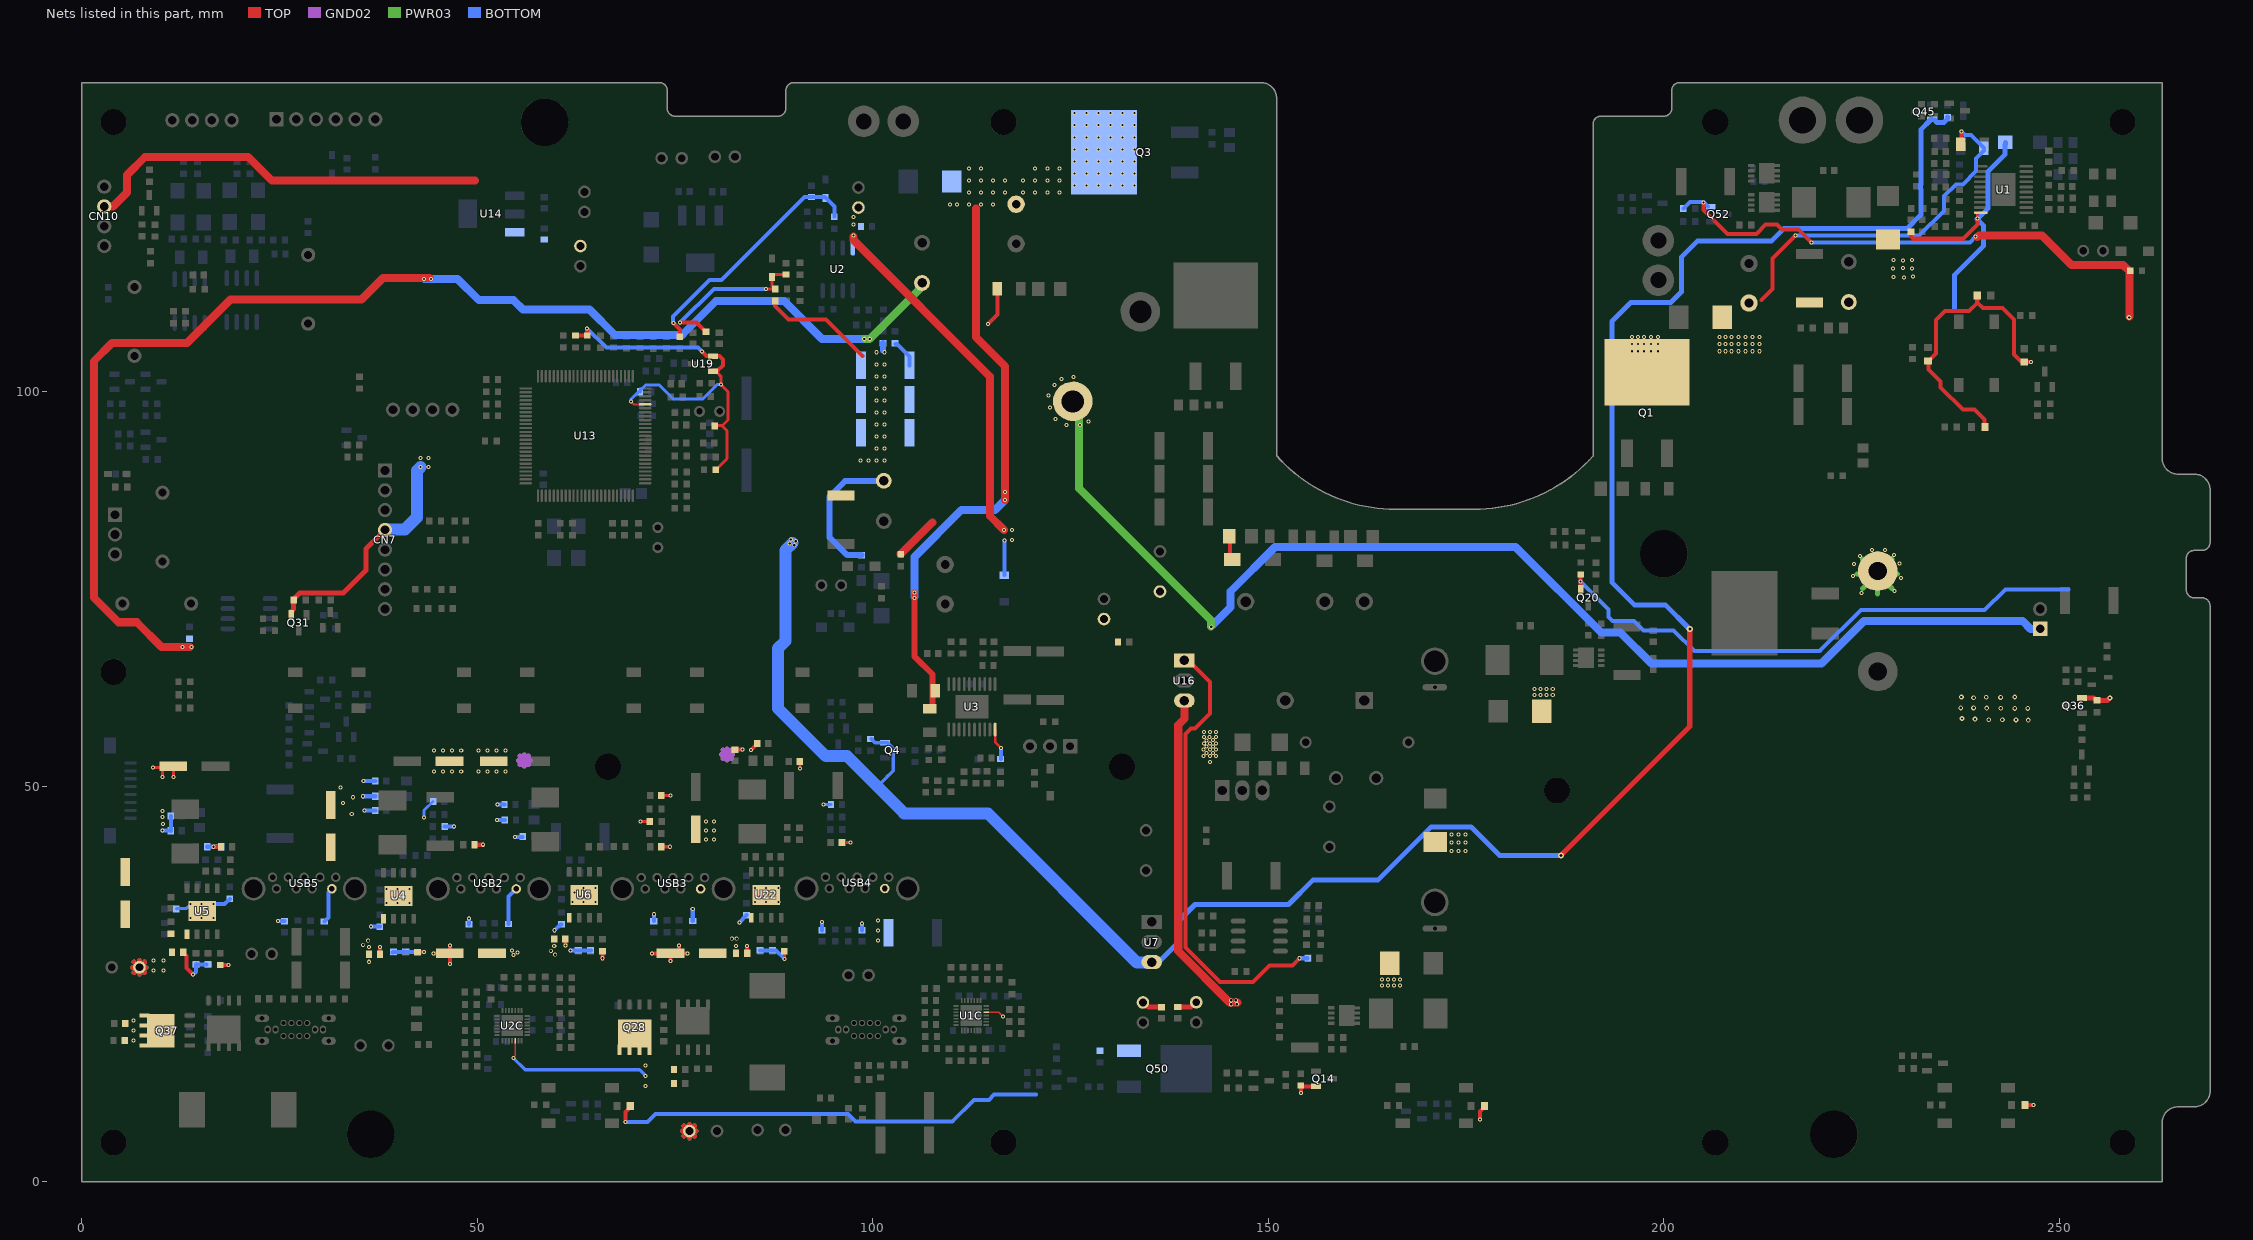
[diagram p0: the nets of this part, all layers, seen from the top]
# Altium PCB MISC84402.PcbDoc (part 3 of 12)
Units mm, origin at the board's own origin, x right, y up, seen from the top; angles counter-clockwise.
Board outline 269.06 x 139 mm, 4 copper layers (TOP, GND02, PWR03, BOTTOM), stack 0.732 mm thick; 694 components, 428 nets, 1859 pads, 1384 vias.

## Footprints (in the part's own frame and the unit in brackets; to place one, negate y for a bottom-side part, rotate by r counter-clockwise, add the part's x,y. Pads: shape width x height; smd on the part's side, far side on the other; paste and mask are expansions set on the pad) (continued)
SOD-123FL_L2.7-W1.8-LS3.8-RD [mm]
  rect 1.4x1.2 smd: 1(-1.735,0) 2(1.735,0)
  silkscreen extent -1.6,-1 1.38,1
SOD-323_L1.8-W1.3-LS2.5-RD [mm]
  rect 1x0.75 smd: 1(-1.173,0) 2(1.173,0)
  silkscreen extent -1.08,-0.8 0.9,0.8
SOIC-8_L5.0-W4.0-P1.27-LS6.0-BL [mm]
  oval 0.568x1.95 smd: 1(-2.59,-1.623) 2(-1.32,-1.623) 3(-0.05,-1.623) 4(1.22,-1.623) 5(1.22,3.787) 6(-0.05,3.787) 7(-1.32,3.787) 8(-2.59,3.787)
  silkscreen extent -3.38,-1.73 1.81,2.99
SOP-8_L4.9-W3.9-P1.27-LS6.0-BL [mm]
  oval 0.63x1.865 smd: 1(-1.905,-2.682) 2(-0.635,-2.682) 3(0.635,-2.682) 4(1.905,-2.682) 5(1.905,2.683) 6(0.635,2.683) 7(-0.635,2.683) 8(-1.905,2.683)
  silkscreen extent -2.82,-2.83 2.58,1.52
SOP-8_L5.0-W4.0-P1.27-LS6.0-BL [mm]
  oval 0.574x2.036 smd: 1(-1.905,-2.768) 2(-0.635,-2.768) 3(0.635,-2.768) 4(1.905,-2.768) 5(1.905,2.768) 6(0.635,2.768) 7(-0.635,2.768) 8(-1.905,2.768)
  silkscreen extent -2.79,-2.92 2.53,1.52
SOT-23-3_L2.9-W1.3-P1.90-LS2.4-BR [mm]
  rect 1.25x0.7 smd: 1(1,-0.95) 2(1,0.95) 3(-1,0)
  silkscreen extent -0.73,-1.53 0.73,1.53
SOT-23-3_L2.9-W1.6-P1.90-LS2.8-BR-CW [mm]
  rect 1.25x0.7 smd: 1(1.25,-0.95) 2(-1.25,0) 3(1.25,0.95)
  silkscreen extent -0.76,-1.52 0.89,1.52
SOT-223-3_L6.5-W3.4-P2.30-LS7.0-BR [mm]
  rect 2.5x1.1 smd: 1(2.97,-2.3) 2(2.97,0) 3(2.97,2.3)
  rect 2.34x3.6 smd: 4(-2.97,0)
  silkscreen extent -1.57,-3.33 1.37,3.33
SW-SMD_4P-L6.0-W6.0-P4.50-LS8.6 [mm]
  rect 1.8x1.2 smd: 1(-4,2.25) 2(4,2.25) 3(-4,-2.25) 4(4,-2.25)
  silkscreen extent -3,-3 3,3
TO-92-3_L4.8-W3.7-P2.54-L [mm]
  rect 1.8x1.8 hole 1: 1(-2.54,0)
  round 1.8 hole 1: 2(0,0) 3(2.54,0)
  silkscreen extent -2.17,-1.5 2.14,2.48
TO-220-3_L10.0-W4.5-P2.54-L [mm]
  rect 1.8x2.6 hole 1.2: 1(-2.54,0.005)
  oval 1.8x2.6 hole 1.2: 2(0,0.005) 3(2.54,-0.005)
  silkscreen extent -5.3,-2.73 5.3,3.09
TO-252-2_L6.6-W6.1-P4.57-LS9.9-BR [mm]
  rect 1.6x3 smd: 1(-2.285,-4.806) 2(2.285,-4.8)
  rect 6x6.5 smd: 3(0,2.428)
  silkscreen extent -3.57,-3.07 3.57,6.18
TO-263-3_L10.2-W10.7-P5.08-LS16.2-TL [mm]
  rect 3.504x1.5 smd: 1(-6.326,2.54) 3(-6.326,-2.54)
  rect 8.38x10.7 smd: 2(3.888,0)
  silkscreen extent -4.11,-5 -1.51,5
USB-A-TH_916-252A205IY30200 [mm]
  round 1.2 hole 0.7: 1(-3.5,-0.72) 2(-1,-0.72) 3(1,-0.72) 4(3.5,-0.72) 5(4,0.72) 6(2,0.72) 7(0,0.72) 8(-2,0.72) 9(-4,0.72)
  round 3 hole 2.3: 10(-6.4,-0.72) 11(6.4,-0.72)
  silkscreen extent -7.24,-3.68 7.24,2.29

## Part data
U1C U2C: library part SW3516

## Free pads (board coordinates)
  round 3.3 / inner round 1.524 / far side round 1.524 hole 3.3: 0(3.98,134)
  round 3.3 / inner round 1.524 / far side round 1.524 hole 3.3 unplated: 0(4,64.5) 0(4,5) 0(66.5,52.5) 0(116.5,5) 0(116.5,134) 0(131.5,52.5) 0(186.5,49.5) 0(206.5,5) 0(206.5,134) 0(258,5) 0(258,134)
  round 6 hole 6 unplated: 0(36.5,6.03) 0(58.5,134) 0(200,79.41)
  round 6 / inner round 1.524 / far side round 1.524 hole 6 unplated: 0(221.5,6.03)

## Via types
v1: diameter 0.508, hole 0.254, TOP to BOTTOM, tented both sides, 1015 vias
v2: diameter 0.508, hole 0.254, TOP to BOTTOM, 243 vias
v3: diameter 0.508, hole 0.305, TOP to BOTTOM, 60 vias
v4: diameter 0.61, hole 0.305, TOP to BOTTOM, 55 vias
v5: diameter 0.61, hole 0.305, TOP to BOTTOM, tented both sides, 8 vias
v6: diameter 0.762, hole 0.381, TOP to BOTTOM, 2 vias
v7: diameter 0.762, hole 0.381, TOP to BOTTOM, tented both sides, 1 vias

## Nets (pads, with @x,y where several pads share a name; then routed paths per layer and width w, separated by ;. In a path a pad name is that pad's centre, name@x,y a point inside that pad or via, vN(x,y) a via of type N, cw(c..) or ccw(c..) an arc to the next point about the centre after c; other vN are vias at no path point)
2.5V: C39.2 R33.2 R46.2 R224.1 R269.1 U13.21 U19.1 U19.3 | length 53.8
  TOP w0.254: v1(69.395,98.671) 69.74,98.326 U13.21@71.203,98.326
  TOP w0.381: R46.2@80.027,95.596 R46.2@80.112,95.596 ; R46.2@80.112,95.631 80.975,95.631 81.686,96.342 81.686,99.898 v1@80.848,100.736 ; U19.1@80.289,102.362 80.772,101.879 v1@80.772,100.829 ; R33.2@80.366,90.246 81.56,91.441 81.56,94.961 80.925,95.596 ; 80.391,102.514 80.416,102.489 ; v1(80.798,100.803) v1@80.856,100.744
  TOP w0.508: R224.1@62.383,107.017 R269.1@63.881,107.017 v1(63.881,107.915) ; v1(78.385,104.994) 78.959,104.42 U19.3@79.762,104.42 80.619,104.42 81.026,104.013 81.026,103.251 80.34,102.565 U19.1@79.883,102.565
  BOTTOM w0.381: v1(69.395,98.671) 69.395,98.925 70.384,99.914 C39.2@70.573,99.914 ; C39.2@70.637,99.873 C39.2@70.637,100.254 ; C39.2@70.79,100.254 71.323,100.787 72.949,100.787 74.727,99.009 78.511,99.009 80.315,100.813 v1@80.747,100.813
  BOTTOM w0.508: v1(63.881,107.915) 66.294,105.502 77.877,105.502 v1(78.385,104.994)
13.6V-I: C43.2 D12.1 R147.2 R317.2 | length 31.2
  TOP w0.508: v2(74.778,108.585) 75.59,107.772 R317.2@75.59,107.036
  BOTTOM w0.508: v2(74.778,108.585) 74.752,108.585 74.752,109.449 79.324,114.021 80.848,114.021 91.364,124.536 93.929,124.536 95.123,123.342 R147.2@95.123,122.038
13.6V-U: C159.1 D41.1 R86.2 R295.1 | length 21.1
  TOP w0.254: v2(75.641,108.661) v2@75.743,108.661
  TOP w0.381: v1(86.487,112.903) R295.1@87.639,112.903 87.249,113.293 D41.1@87.249,114.397 87.595,114.743 C159.1@89,114.743
  TOP w0.508: v2@75.743,108.661 77.715,108.661 R86.2@78.892,107.484
  BOTTOM w0.381: v2(75.641,108.661) v2@75.641,108.687
  BOTTOM w0.508: v2(75.641,108.661) 79.908,112.928 v1@86.487,112.928
+5V: C9.2 C28.1 C30.1 C76.1 C152.1 C167.1 Q4.2 Q45.2 Q50.2 R291.1 R314.1 R351.1 U7.3 U14.3 | length 299.2
  TOP w0.635: C30.1@134.544,22.377 134.819,22.102 C28.1@136.51,22.102 ; C167.1@138.547,22.113 140.197,22.113 C76.1@140.691,22.606 ; v6(186.995,41.3) 203.276,57.582 v6(203.276,69.901)
  BOTTOM w0.457: R291.1@99.822,56.007 100.279,55.55 101.854,55.55 102.559,54.845 102.559,51.988 102.184,51.613 ; 100.914,50.343 102.184,51.613 ; 101.829,51.257 102.184,51.613 ; 102.248,51.676 102.184,51.613
  BOTTOM w0.635: U7.3@136.246,27.915 138.506,30.175 138.506,32.868 140.716,35.077 152.552,35.077 155.626,38.151 163.83,38.151 170.586,44.907 175.616,44.907 179.222,41.3 v6(186.995,41.3) ; v6@203.124,70.028 200.228,72.923 196.317,72.923 193.421,75.819 193.421,108.788 195.834,111.201 200.889,111.201 202.209,112.522 202.209,116.916 204.241,118.948 213.589,118.948 215.163,120.523 230.734,120.523 232.486,122.276 232.486,125.504 232.474,125.517 232.474,126.096 232.486,126.108 232.486,133.045 233.78,134.339 Q45.2@233.902,134.339 ; v6@203.136,70.04 v6(203.276,69.901) ; Q45.2@234.239,134.264 234.544,133.96 235.407,133.96 235.881,134.433 R314.1@235.881,134.62
  BOTTOM w1.524: 89.84,80.772 88.925,79.858 88.925,68.377 87.986,67.437 87.986,59.893 94.046,53.832 96.738,53.832 103.961,46.609 114.529,46.609 133.401,27.737 U7.3@135.077,27.737 ; U7.3@135.077,27.796 U7.3@135.244,27.796
  other v3: 90.068,80.518 89.484,80.721 90.246,81.026 89.637,81.229
+12V: C65.1 C96.1 CN7.4 CN10.3 LED1.1 LED2.1 LED3.1 LED4.1 LED5.1 LED6.1 LED7.1 Q14.2 Q20.2 Q31.2 Q36.2 Q52.2 R23.1 R35.1 R48.2 R98.1 R289.1 R353.1 R362.1 U16.3 | length 372.1
  TOP w0.508: v2(68.732,7.595) 68.732,8.839 LED3.1@69.19,9.296 ; R23.1@154.07,12.097 Q14.2@156.032,12.097 ; v2(154.102,11.227) R23.1@154.102,12.191 ; v2(176.759,7.874) 176.759,8.89 LED4.1@177.292,9.423 ; v2(189.459,75.921) v2@189.484,75.921 ; Q20.2@189.484,75.261 v2@189.484,75.921 ; R35.1@189.484,76.808 v2@189.484,75.921 ; v2(205.019,123.86) 205.019,122.895 208.051,119.863 211.684,119.863 212.877,121.056 214.3,121.056 214.909,120.447 217.018,120.447 v2(218.669,118.796) ; LED5.1@233.384,103.79 233.457,103.79 234.417,104.75 234.417,108.991 235.534,110.109 238.531,110.109 ; LED5.1@233.451,103.759 233.451,102.743 235.001,101.194 235.001,100.457 237.795,97.663 239.293,97.663 240.563,96.393 LED6.1@240.563,95.682 ; 238.608,110.109 239.624,111.125 ; LED7.1@239.624,111.963 239.624,111.201 240.335,110.49 242.799,110.49 244.246,109.042 244.246,104.648 LED2.1@245.288,103.607 ; LED2.1@245.364,103.671 v2(246.419,103.671) ; LED1.1@245.618,9.754 v2(246.761,9.754)
  TOP w0.61: Q36.2@252.85,61.19 254.328,61.19 254.635,60.884 256.083,60.884 v4(256.388,61.189)
  TOP w0.635: Q31.2@26.49,71.697 26.49,72.134 26.772,72.415 26.772,73.711 27.534,74.473 33.045,74.473 35.89,77.318 35.89,80.035 CN7.4@38.024,82.169
  TOP w1.016: CN10.3@2.819,123.339 3.934,123.339 5.69,125.095 5.69,127.305 8.001,129.616 21.006,129.616 24.003,126.619 49.682,126.619 ; R362.1@103.521,79.375 107.509,83.363 ; U16.3@139.388,60.858 139.388,58.565 138.608,57.785 138.608,29.185 145.085,22.708 v3@146.075,22.708 ; v2@239.624,119.456 239.827,119.659 241.148,119.659 ; 240.538,119.659 241.148,119.659 ; v4@258.851,109.398 258.851,115.164 258.064,115.951 251.536,115.951 247.828,119.659 241.148,119.659
  BOTTOM w0.508: v2(68.732,7.595) 71.501,7.595 72.517,8.611 96.825,8.611 97.79,7.645 110.033,7.645 112.776,10.389 114.264,10.389 ; 114.267,10.392 114.659,10.392 115.341,11.074 120.65,11.074 ; v2(189.459,75.921) 189.459,75.895 192.989,72.365 192.989,71.45 193.523,70.917 196.215,70.917 197.409,69.723 201.244,69.723 203.86,67.107 219.71,67.107 224.917,72.314 240.563,72.314 243.18,74.93 251.13,74.93 ; R353.1@202.464,123.072 203.277,123.885 v2@205.019,123.885 ; v2(205.019,123.86) v2@205.019,123.885 ; Q52.2@205.562,123.342 v2@205.019,123.885 ; v2(218.669,118.796) 238.709,118.796 v2(239.42,119.507)
  BOTTOM w1.524: CN7.4@38.465,82.487 40.823,82.487 42.365,84.029 42.365,89.928 v1(42.825,90.389)
  other v1: 43.841,90.389 42.825,91.532 43.841,91.532
  other v3: 145.288,22.454 146.025,22.479 145.288,22.962 145.898,22.962
  other v4: 258.826,109.296
+13.6V: C6.1 F2.1 F3.1 F4.1 R75.2 R106.2 R108.2 R109.2 R210.1 R268.1 R326.2 R358.2 U3.10 | length 37.8
  TOP w0.305: U3.10@115.447,56.458 U3.10@115.447,57.198 115.447,55.622 v1(116.187,54.882)
  TOP w0.508: R75.2@87.639,111.379 87.639,110.761 89.332,109.068 94.082,109.068 98.704,104.445
  BOTTOM w0.508: R210.1@116.187,53.449 v1(116.187,54.882)
  BOTTOM w0.762: R326.2@98.552,79.239 96.783,79.239 94.539,81.483 94.539,86.665 96.495,88.621 C6.1@101.168,88.621 ; C6.1@101.284,88.504 C6.1@101.386,88.606 ; 101.295,105.105 R268.1@101.295,106.054
  other v1: 164.364,24.857 165.126,24.857 165.888,24.857 166.65,24.857 164.364,25.619 165.126,25.619 165.888,25.619 166.65,25.619 142.621,53.086 141.808,53.848 142.596,53.848 143.383,53.848 141.808,54.686 142.596,54.686 143.358,54.686 141.834,55.448 142.596,55.448 143.383,55.448 141.834,56.261 143.358,56.261 142.57,56.286 141.859,56.896 142.621,56.896 143.383,56.896 183.668,61.56 184.43,61.56 185.192,61.56 185.954,61.56 183.668,62.322 184.43,62.322 185.192,62.322 185.954,62.322 98.425,91.186 99.441,91.186 100.457,91.186 101.473,91.186 100.457,92.71 101.473,92.71 100.457,94.234 101.473,94.234 100.457,95.758 101.473,95.758 100.457,97.282 101.473,97.282 100.457,98.806 101.473,98.806 100.457,100.33 101.473,100.33 100.457,101.854 101.473,101.854 100.457,103.378 101.473,103.378 100.457,104.902 101.473,104.902
  other v2: 142.164,54.254 143.002,54.254 142.189,55.042 142.977,55.067 142.189,55.829 143.002,55.855 230.353,114.351 229.057,114.427 231.47,114.452 228.981,115.468 231.369,115.519 230.226,115.545 230.251,116.51 231.369,116.535 229.032,116.561
  other v4: 246.075,58.395 244.526,58.42 241.071,58.445 242.799,58.445 239.344,58.522 237.693,58.598 244.373,59.868 245.999,59.868 242.595,59.893 240.817,59.919 237.541,59.944 239.166,59.944 239.166,61.214 242.57,61.265 240.767,61.29 237.617,61.316 244.373,61.316
+13.6V-F: C112.1 CON1.1 L1.2 R106.1 R108.1 R109.1 R197.1 R198.2 R281.1 | length 327.8
  TOP w0.508: v1(114.554,108.458) 115.742,109.646 R198.2@115.742,112.903
  TOP w1.016: v1@13.691,67.656 v1(12.7,67.656) 10.043,67.656 6.934,70.764 4.623,70.764 1.499,73.889 1.499,103.759 3.81,106.07 13.284,106.07 18.771,111.557 35.331,111.557 38.075,114.3 v1@43.967,114.3
  PWR03 w1.016: v4@98.984,106.553 99.568,106.553 C112.1@106.248,113.233 ; L1.2@125.276,98.697 126.086,97.887 126.086,87.681 142.773,70.993 v4@142.773,70.256
  BOTTOM w0.508: R281.1@102.87,105.927 103.064,105.927 104.648,104.343 R109.1@104.648,103.251
  BOTTOM w1.016: v1@43.282,114.173 v1(44.12,114.173) 47.498,114.173 50.19,111.481 54.559,111.481 55.753,110.287 64.186,110.287 67.361,107.112 75.895,107.112 80.188,111.404 88.748,111.404 93.574,106.578 v4(98.908,106.578) v4@99.466,106.578 ; v4@142.875,70.333 145.237,72.695 145.237,74.676 150.851,80.289 181.254,80.289 192.1,69.444 194.513,69.444 198.425,65.532 219.939,65.532 225.323,70.917 245.37,70.917 246.361,69.926 CON1.1@247.574,69.926 ; CON1.1@247.421,70.002 CON1.1@247.955,70.002
  other v1: 13.869,67.656 43.231,114.173
  other v2: 124.46,95.682 126.162,95.682 127.279,96.164 123.088,96.444 122.377,97.892 122.199,99.441 122.987,100.736 123.876,101.549 125.374,101.752
  other v4: 142.773,70.18 99.593,106.578
+24V: C4.1 C23.1 C55.2 C60.2 C63.1 C64.1 C79.2 C97.1 C140.1 C147.2 C161.2 C162.2 C172.1 C176.2 C399.2 D50.1 L2.2 Q28.5 Q28.6 Q28.7 Q28.8 Q37.5 Q37.6 Q37.7 Q37.8 R136.2 R273.1 R277.1 R278.1 R279.1 R367.2 U1.10 U1C.19 U2C.19 U4.5 U5.5 U6.5 U22.5 | length 111
  TOP w0.203: v1@54.559,15.773 54.782,15.996 U2C.19@54.782,17.869 ; U1C.19@114.328,21.447 115.894,21.447 v1(116.421,20.92)
  TOP w0.254: v1(54.54,15.682) v1@54.595,15.737
  TOP w0.305: v1(239.649,121.793) 239.649,122.428 239.772,122.551 U1.10@240.078,122.551
  TOP w0.508: R136.2@231.267,120.151 231.267,119.507 231.521,119.253 237.871,119.253 239.649,121.031 v1(239.649,121.793)
  TOP w0.635: 6.413,27.143 C140.1@7.265,27.143 ; 6.612,26.49 C140.1@7.265,27.143 ; 6.612,27.795 C140.1@7.265,27.143 ; 7.265,26.291 C140.1@7.265,27.143 ; 7.265,27.994 C140.1@7.265,27.143 ; 7.918,26.49 C140.1@7.265,27.143 ; 7.918,27.795 C140.1@7.265,27.143 ; 8.116,27.143 C140.1@7.265,27.143 ; 75.938,6.442 C97.1@76.79,6.442 ; 76.137,5.789 C97.1@76.79,6.442 ; 76.137,7.094 C97.1@76.79,6.442 ; 76.79,5.59 C97.1@76.79,6.442 ; 76.79,7.293 C97.1@76.79,6.442 ; 77.443,5.789 C97.1@76.79,6.442 ; 77.443,7.094 C97.1@76.79,6.442 ; 77.641,6.442 C97.1@76.79,6.442
  PWR03 w0.635: 6.413,27.143 C140.1@7.265,27.143 ; 6.612,26.49 C140.1@7.265,27.143 ; 6.612,27.795 C140.1@7.265,27.143 ; 7.265,26.291 C140.1@7.265,27.143 ; 7.265,27.994 C140.1@7.265,27.143 ; 7.918,26.49 C140.1@7.265,27.143 ; 7.918,27.795 C140.1@7.265,27.143 ; 8.116,27.143 C140.1@7.265,27.143 ; 75.938,6.442 C97.1@76.79,6.442 ; 76.137,5.789 C97.1@76.79,6.442 ; 76.137,7.094 C97.1@76.79,6.442 ; 76.79,5.59 C97.1@76.79,6.442 ; 76.79,7.293 C97.1@76.79,6.442 ; 77.443,5.789 C97.1@76.79,6.442 ; 77.443,7.094 C97.1@76.79,6.442 ; 77.641,6.442 C97.1@76.79,6.442 ; 224.449,76.876 L2.2@227.001,76.876 ; 225.146,75.021 L2.2@227.001,76.876 ; L2.2@225.146,78.731 L2.2@227.001,76.876 ; 227.001,74.324 L2.2@227.001,76.876 ; L2.2@227.001,79.427 L2.2@227.001,76.876 ; 228.856,75.021 L2.2@227.001,76.876 ; L2.2@228.856,78.731 L2.2@227.001,76.876 ; 229.552,76.876 L2.2@227.001,76.876
  BOTTOM w0.381: v1(54.54,15.682) 56.033,14.189 70.511,14.189 v1(71.273,13.427)
  BOTTOM w0.508: v2(36.551,32.284) R277.1@37.659,32.284 ; v2(59.741,31.826) 60.478,32.563 R278.1@60.621,32.563 ; v2(83.109,32.801) R279.1@84.039,33.732
  BOTTOM w0.635: 236.728,110.49 236.728,114.656 240.386,118.313 240.386,120.955 239.674,121.666 v1@239.674,121.818 ; v1@239.611,121.755 v1(239.649,121.793) v1@239.674,121.818 ; v1@239.725,121.869 v1@239.674,121.818 ; v1@239.751,121.844 241.008,123.101 241.008,127.775 243.154,129.921 D50.1@243.154,131.064 ; D50.1@243.116,131.102 243.172,131.158 D50.1@243.172,131.445
  other v1: 71.273,12.157 71.273,14.697 6.503,17.872 6.503,19.142 6.503,20.412 9.043,26.762 10.313,26.762 36.283,27.842 9.043,28.032 10.313,28.032 36.283,29.683 59.713,29.81 82.7,29.81
  other v2: 54.534,28.677 55.067,29.007 54.356,29.235 224.993,74.473 229.159,74.701 229.972,76.352 223.901,76.606 224.028,78.105 229.794,78.207 224.815,79.121 229.108,79.299 226.339,79.883 227.94,79.883
  other v3: 59.817,28.753 59.284,29.21 35.56,29.972 36.195,30.505 82.169,30.759 82.779,30.759
+VCC_BAT: C44.1 C54.1 C116.1 C154.1 D18.2 D62.1 R155.1 U2.8 U16.1 | length 109.5
  TOP w0.508: U16.1@139.378,65.938 139.929,65.938 142.629,63.238 142.629,59.241 140.716,57.328 140.208,57.328 139.548,56.667 139.548,29.642 143.891,25.298 144.475,25.298 148.057,25.298 150.134,27.376 153.04,27.376 v1(153.95,28.286) ; D62.1@145.136,79.4 145.141,79.406 C154.1@145.141,81.518
  TOP w1.016: v1@97.536,119.507 97.536,119.101 114.783,101.854 114.783,84.226 v1(116.586,82.423)
  BOTTOM w0.508: D18.2@116.612,76.714 v1(116.612,81.127) ; v1(153.95,28.286) R155.1@154.975,28.286
  other v1: 117.602,81.153 117.602,82.423 97.536,119.634 97.536,121.031 97.536,122.022
AGND: C23.2 C29.1 C31.1 C46.1 C49.1 C57.1 C60.1 C62.1 C63.2 C64.2 C77.2 C92.1 C95.2 C101.1 C102.1 C105.1 C106.1 C114.1 C117.1 C122.2 C123.1 C142.1 C144.1 C147.1 C150.1 C153.1 C160.2 C161.1 C162.1 C165.1 C166.1 C169.1 C170.1 C172.2 C173.1 C174.1 C175.1 C177.1 C180.1 C181.1 C182.1 C183.1 C184.1 C185.1 C186.1 C187.1 C192.1 C199.1 R24.1 R30.1 R58.1 R59.2 R77.2 R85.1 R132.1 R133.1 R135.1 R292.1 U4.9 U5.9 U6.9 U22.9 USB2.4 USB3.4 USB4.4 USB5.4 | length 110.9
  TOP w0.381: v1(8.966,52.375) C77.2@10.109,52.375 ; v1(10.16,51.181) 10.16,52.197 10.541,52.578 C77.2@11.554,52.578 ; v1(11.557,51.181) 11.554,51.184 C77.2@11.554,52.578 ; C77.2@12.954,52.324 12.7,52.578 C77.2@11.554,52.578 ; v1(70.638,45.558) R58.1@71.79,45.558 ; C170.1@73.243,42.383 v1(74.321,42.383) ; C29.1@73.243,48.86 v1(74.387,48.86) ; v1(88.799,28.22) R292.1@88.799,29.183 ; v1(90.769,52.289) C150.1@90.769,53.178 ; C199.1@96.077,42.926 v1(97.155,42.926)
  TOP w0.508: C147.1@12.791,29.048 12.791,29.018 13.208,28.6 13.208,27.051 v2(14.046,26.213) ; v1(16.663,42.383) C62.1@17.549,42.383 ; R132.1@17.479,27.427 17.509,27.457 v1@18.517,27.457 ; C60.1@37.683,28.794 v2(37.683,29.729) ; R133.1@42.444,29.065 v2(43.238,29.065) ; v2(44.44,28.915) C64.2@46.505,28.915 ; v2(46.505,27.587) C64.2@46.505,28.915 ; v2(46.505,29.893) C64.2@46.505,28.915 ; C49.1@49.621,42.637 v1(50.699,42.637) ; v2(61.113,29.895) C161.1@61.113,30.699 ; v1(65.812,28.286) R135.1@65.812,29.192 ; v2(72.075,28.915) C172.2@74.419,28.915 ; v2(74.419,27.943) C172.2@74.419,28.915 ; v2(75.479,29.886) 75.479,28.915 C172.2@74.419,28.915 ; v2(76.566,28.915) C172.2@74.419,28.915 ; C153.1@82.566,54.658 v2(83.544,54.658) ; C162.1@84.1,28.921 v2(84.1,29.845) ; v2(84.582,54.585) 85.372,55.375 C123.1@85.372,55.439
  GND02 w0.635: 55.221,53.305 55.922,53.305 ; 55.375,52.758 55.922,53.305 ; 55.375,53.851 55.922,53.305 ; 55.922,52.603 55.922,53.305 ; 55.922,54.006 55.922,53.305 ; 56.469,52.758 55.922,53.305 ; 56.469,53.851 55.922,53.305 ; 56.623,53.305 55.922,53.305 ; 80.875,54.067 81.576,54.067 ; 81.029,53.52 81.576,54.067 ; 81.029,54.613 81.576,54.067 ; 81.576,53.365 81.576,54.067 ; 81.576,54.768 81.576,54.067 ; 82.123,53.52 81.576,54.067 ; 82.123,54.613 81.576,54.067 ; 82.277,54.067 81.576,54.067
  PWR03 w0.635: 55.221,53.305 55.922,53.305 ; 55.375,52.758 55.922,53.305 ; 55.375,53.851 55.922,53.305 ; 55.922,52.603 55.922,53.305 ; 55.922,54.006 55.922,53.305 ; 56.469,52.758 55.922,53.305 ; 56.469,53.851 55.922,53.305 ; 56.623,53.305 55.922,53.305 ; 80.875,54.067 81.576,54.067 ; 81.029,53.52 81.576,54.067 ; 81.029,54.613 81.576,54.067 ; 81.576,53.365 81.576,54.067 ; 81.576,54.768 81.576,54.067 ; 82.123,53.52 81.576,54.067 ; 82.123,54.613 81.576,54.067 ; 82.277,54.067 81.576,54.067
  BOTTOM w0.381: R77.2@11.936,34.518 12.012,34.595 13.233,34.595 v1@13.716,35.077 ; v1(43.256,46.101) 43.256,46.99 C46.1@44.374,48.108 ; v1(93.741,47.717) C31.1@94.703,47.717 ; R85.1@96.13,42.926 v1(97.155,42.926)
  BOTTOM w0.508: v2@10.202,44.425 C101.1@11.281,44.425 ; C101.1@11.23,44.399 C102.1@11.23,46.288 ; v2@14.072,26.238 14.412,26.578 C92.1@14.412,27.52 ; C92.1@14.476,27.584 C92.1@14.412,27.52 ; C165.1@15.76,27.52 C92.1@14.412,27.52 ; C144.1@15.839,42.383 v1(16.663,42.383) C192.1@17.614,42.383 ; v1(16.663,35.144) 18.042,35.144 R30.1@18.695,35.796 ; v2(24.762,32.966) C183.1@25.587,32.966 ; C182.1@30.642,32.941 30.68,32.941 31.166,33.426 31.166,36.576 USB5.4@31.547,36.957 ; v2(35.56,48.768) C57.1@37.095,48.768 ; v2(35.62,50.708) C105.1@37.087,50.708 ; v2(35.722,46.948) C106.1@37.087,46.948 ; C166.1@39.243,29.007 39.319,29.083 41.148,29.083 41.166,29.065 v2(43.238,29.065) ; C169.1@40.745,29.111 C169.1@40.767,29.134 ; R24.1@45.855,44.923 v1(47.016,44.923) ; C185.1@48.955,32.585 v2(48.955,33.29) ; v2(52.493,45.755) C117.1@53.47,45.755 ; v2(52.562,47.71) C114.1@53.419,47.71 ; C184.1@53.933,32.611 53.933,36.103 USB2.4@54.686,36.855 ; v1(54.75,43.616) C142.1@55.702,43.616 ; v2(61.75,29.289) C173.1@62.754,29.289 C174.1@64.364,29.289 ; C180.1@72.298,32.966 v2(72.298,33.849) ; C181.1@77.225,32.992 v2(77.225,34.484) ; C175.1@85.741,29.289 87.754,29.289 v1@88.748,28.296 ; C187.1@93.583,31.823 v2(93.583,32.884) ; C186.1@98.612,31.823 v2(98.612,32.706)
  other v1: 18.542,27.457 100.661,30.546 100.661,31.816 100.661,33.086 13.742,33.366 15.139,33.366 16.663,33.366 13.742,35.144 15.139,35.144 38.507,35.271 39.904,35.271 41.428,35.271 62.002,35.398 63.399,35.398 64.923,35.398 85.116,35.398 86.513,35.398 88.037,35.398 62.256,36.617 38.507,37.049 39.904,37.049 41.428,37.049 63.399,37.176 64.923,37.176 85.116,37.176 86.513,37.176 88.037,37.176 78.918,43.282 79.934,43.282 78.918,44.425 79.934,44.425 78.918,45.568 79.934,45.568 44.526,51.918 45.669,51.918 46.812,51.918 47.955,51.918 50.111,51.918 51.254,51.918 52.397,51.918 53.54,51.918 44.526,54.559 45.669,54.559 46.812,54.559 47.955,54.559 50.111,54.559 51.254,54.559 52.397,54.559 53.54,54.559
  other v2: 10.211,44.425 10.242,45.257 10.205,46.171 34.112,46.507 10.169,46.905 33.02,47.93 34.265,48.641 32.69,49.86
B+: C38.1 C128.1 F1.2 F5.2 F6.1 Q1.2 Q3.2 R1.2 R54.2 R330.2 R331.2 | length 120.2
  TOP w0.508: 212.319,111.481 213.741,112.903 213.741,116.738 v1@216.586,119.583 ; v1@216.599,119.57 v1(216.662,119.634) ; R1.2@237.535,131.191 237.617,131.273 v1(237.617,132.842)
  TOP w0.762: v1@105.283,74.498 105.283,66.421 107.544,64.16 107.544,59.842 R54.2@107.594,59.792
  TOP w1.016: 113.03,123.063 113.03,106.807 116.713,103.124 v1(116.713,87.249) v1(116.713,86.233)
  BOTTOM w0.508: v1(216.662,119.634) 232.283,119.634 235.433,122.784 235.433,124.638 236.931,126.136 237.82,126.136 239.471,127.787 239.471,129.413 R330.2@240.487,130.429 ; v1@237.592,132.842 238.074,132.359 238.816,132.359 R330.2@240.467,130.708
  BOTTOM w1.016: v1@105.258,73.99 105.258,79.019 111.176,84.938 115.418,84.938 v1(116.713,86.233) v1(116.713,87.249)
  other v1: 173.127,41.875 174.016,41.875 174.905,41.875 173.127,42.891 174.016,42.891 174.905,42.891 173.127,43.907 174.016,43.907 174.905,43.907 105.258,73.812 105.258,74.498 195.961,105.029 196.723,105.029 197.485,105.029 198.374,105.029 199.263,105.029 207.01,105.029 207.772,105.029 208.534,105.029 209.423,105.029 210.312,105.029 211.201,105.029 212.09,105.029 195.961,105.918 196.723,105.918 197.485,105.918 198.374,105.918 199.263,105.918 207.01,105.918 207.772,105.918 208.534,105.918 209.423,105.918 210.312,105.918 211.201,105.918 212.09,105.918 195.961,106.807 196.723,106.807 197.485,106.807 198.374,106.807 199.263,106.807 207.01,106.807 207.772,106.807 208.534,106.807 209.423,106.807 210.312,106.807 211.201,106.807 212.09,106.807 109.728,123.571 110.617,123.571 112.141,123.571 113.665,123.571 115.189,123.571 112.141,125.095 113.665,125.095 115.189,125.095 116.713,125.095 118.999,125.095 120.523,125.095 122.047,125.095 123.571,125.095 125.476,125.984 127,125.984 128.524,125.984 130.048,125.984 131.572,125.984 133.096,125.984 112.141,126.619 113.665,126.619 115.189,126.619 116.713,126.619 118.999,126.619 120.523,126.619 122.047,126.619 123.571,126.619 125.476,127.508 127,127.508 128.524,127.508 130.048,127.508 131.572,127.508 133.096,127.508 112.141,128.143 113.665,128.143 120.523,128.143 122.047,128.143 123.571,128.143 125.476,129.032 127,129.032 128.524,129.032 130.048,129.032 131.572,129.032 133.096,129.032 125.476,130.556 127,130.556 128.524,130.556 130.048,130.556 131.572,130.556 133.096,130.556 125.476,132.08 127,132.08 128.524,132.08 130.048,132.08 131.572,132.08 133.096,132.08 125.476,133.604 127,133.604 128.524,133.604 130.048,133.604 131.572,133.604 133.096,133.604 125.476,135.128 127,135.128 128.524,135.128 130.048,135.128 131.572,135.128 133.096,135.128